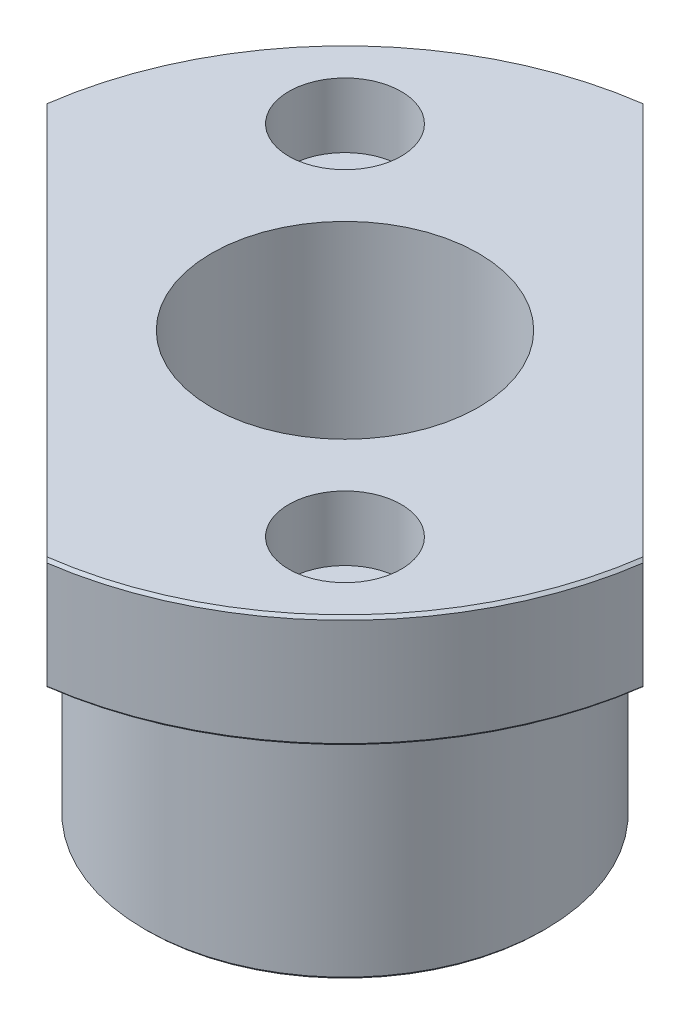
from build123d import *

# Parameters (mm, degrees)
G1_2_TAPPED_HOLE1_D                               = 19
HOLE_SIZE_BASED_ON_SOCKET_HEAD_CAP_SC_D           = 4.8
HOLE_SIZE_BASED_ON_SOCKET_HEAD_CAP_SC_CBORE_D     = 8
HOLE_SIZE_BASED_ON_SOCKET_HEAD_CAP_SC_CBORE_DEPTH = 4.6
CHAMFER1_SIZE                                     = 0.2
CHAMFER2_SIZE                                     = 0.2
SKETCH7_OUTSIDE_W                                 = 67.362
SKETCH7_OUTSIDE_H                                 = 67.362
CUT_EXTRUDE1_DEPTH                                = 50


with BuildPart() as part:
    # Sketch2 → Revolve1 (revolve)
    with BuildSketch(Plane.XY, mode=Mode.PRIVATE) as revolve1_sk:
        Polygon((0, 30), (-25, 30), (-25, 22), (-14.25, 22), (-14.25, 0), (0, 0), align=None)
    revolve(revolve1_sk.sketch.rotate(Axis((0, 0, 0), (0, 1, 0)), 270), axis=Axis((0, 0, 0), (0, 1, 0)))

    # G1/2 Tapped Hole1 (through all)
    with Locations(Plane.ZX.offset(30)):
        with Locations((0, 0)):
            Hole(G1_2_TAPPED_HOLE1_D / 2)

    # Hole Size (% based on) Socket Head Cap Screw Type 1 (through all)
    with Locations(Plane(origin=(-12.727922061, 30, -12.727922061), x_dir=(0, 0, 1), z_dir=(0, 1, 0))):
        with Locations((0, 0), (25.455844122, 25.455844122)):
            CounterBoreHole(HOLE_SIZE_BASED_ON_SOCKET_HEAD_CAP_SC_D / 2, HOLE_SIZE_BASED_ON_SOCKET_HEAD_CAP_SC_CBORE_D / 2, HOLE_SIZE_BASED_ON_SOCKET_HEAD_CAP_SC_CBORE_DEPTH)

    # Chamfer1
    chamfer1_edges = [part.edges().sort_by_distance(p)[0] for p in [
        (0, 0, 14.25),
        (0, 22, 25),
        (0, 30, 25),
    ]]
    chamfer(chamfer1_edges, length=CHAMFER1_SIZE)

    # Chamfer2
    chamfer2_edges = [part.edges().sort_by_distance(p)[0] for p in [
        (0, 22, 14.25),
    ]]
    chamfer(chamfer2_edges, length=CHAMFER2_SIZE)

    # Sketch7 outside → Cut-Extrude1 (cut)
    with BuildSketch(Plane(origin=(0, 30, 0), x_dir=(1, 0, 0), z_dir=(0, 1, 0))):
        Rectangle(SKETCH7_OUTSIDE_W, SKETCH7_OUTSIDE_H)
        Polygon((-24.748737342, 45.961940777), (45.961940777, -24.748737342), (24.748737342, -45.961940777), (-45.961940777, 24.748737342), align=None, mode=Mode.SUBTRACT)
    extrude(amount=-CUT_EXTRUDE1_DEPTH, mode=Mode.SUBTRACT)


solid = part.part
